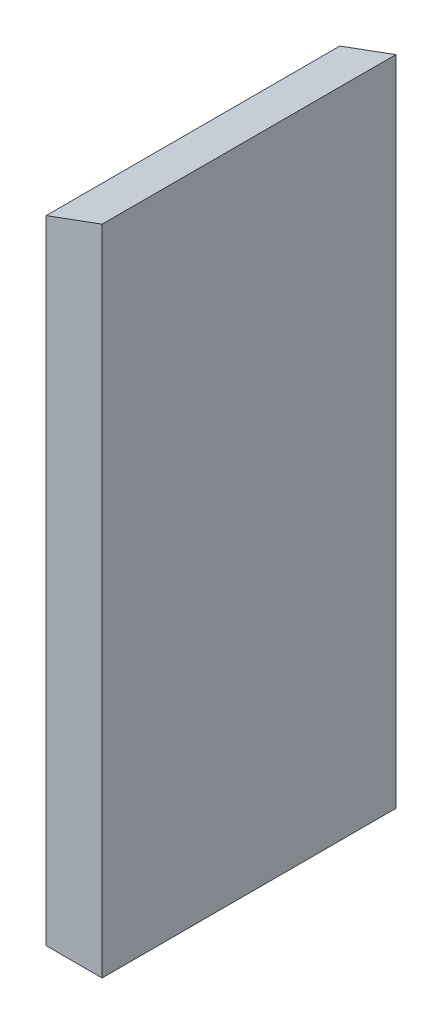
SolidWorks part; units mm, degrees
ref_plane "前视基准面" through (0, 0, 0) normal (0, 0, 1) x (1, 0, 0)
ref_plane "上视基准面" through (0, 0, 0) normal (0, 1, 0) x (1, 0, 0)
ref_plane "右视基准面" through (0, 0, 0) normal (1, 0, 0) x (0, 0, -1)
sketch "草图1" plane through (0, 0, 0) normal (0, 0, 1) x (1, 0, 0)
  line L0 (176.4778, 193) -> (184.4778, 193)
  line L2 (184.4778, 193) -> (184.4778, 286.3582)
  line L4 (184.4778, 286.3582) -> (176.4778, 283.4248)
  line L5 (176.4778, 283.4248) -> (176.4778, 193)
extrude "凸台-拉伸1" add sketch "草图1" along normal blind 25
sketch "草图2" plane through (0, 0, 25) normal (0, 0, 1) x (1, 0, 0)
  line L8 (176.4778, 283.4248) -> (176.4778, 193)
  line L9 (176.4778, 193) -> (184.4778, 193)
  line L10 (184.4778, 193) -> (184.4778, 286.3582)
  line L11 (184.4778, 286.3582) -> (176.4778, 283.4248)
  line L12 (176.4778, 283.4248) -> (176.4778, 193)
  line L13 (176.4778, 193) -> (184.4778, 193)
  line L14 (184.4778, 193) -> (184.4778, 286.3582)
  line L15 (184.4778, 286.3582) -> (176.4778, 283.4248)
  dimension "D1" = 0
extrude "凸台-拉伸2" add sketch "草图2" along normal blind 17
